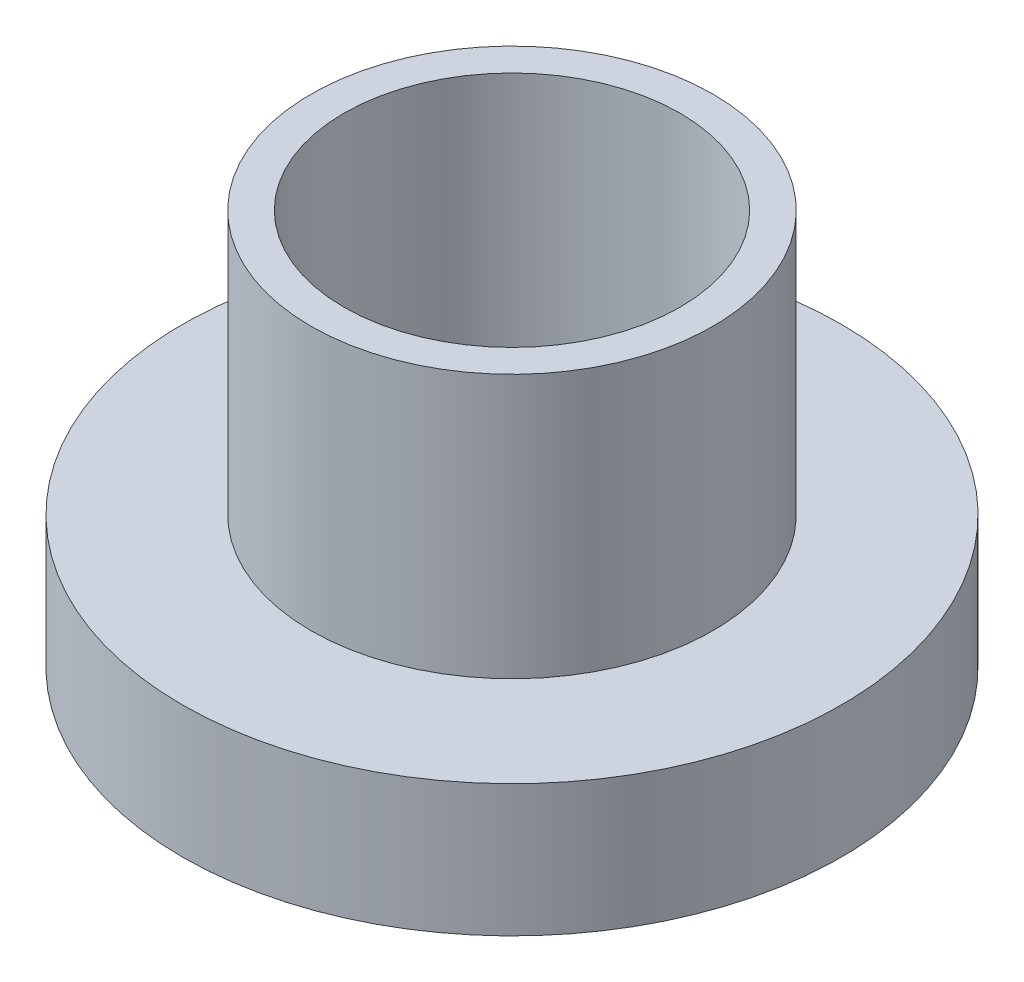
SolidWorks part; units mm, degrees
material "Q235B"
ref_plane "Front Plane" through (0, 0, 0) normal (0, 0, 1) x (1, 0, 0)
ref_plane "Top Plane" through (0, 0, 0) normal (0, 1, 0) x (1, 0, 0)
ref_plane "Right Plane" through (0, 0, 0) normal (1, 0, 0) x (0, 0, -1)
sketch "Sketch1" plane through (0, 0, 0) normal (0, 0, 1) x (1, 0, 0)
  line L0 (0, 0) -> (0, 14.8683) construction
  line L1 (25.5, 60) -> (25.5, 20)
  line L2 (25.5, 20) -> (12.5, 20)
  line L3 (12.5, 20) -> (12.5, 0)
  line L4 (12.5, 0) -> (50, 0)
  line L5 (50, 0) -> (50, 20)
  line L6 (50, 20) -> (30.5, 20)
  line L7 (30.5, 20) -> (30.5, 60)
  line L8 (30.5, 60) -> (25.5, 60)
  dimension "D1" = 61
  dimension "D2" = 51
  dimension "D3" = 25
  dimension "D4" = 100
  dimension "D5" = 60
  dimension "D6" = 20
  dimension "D7" = 20
revolve "Revolve1" add sketch "Sketch1" angle 360 about L0
